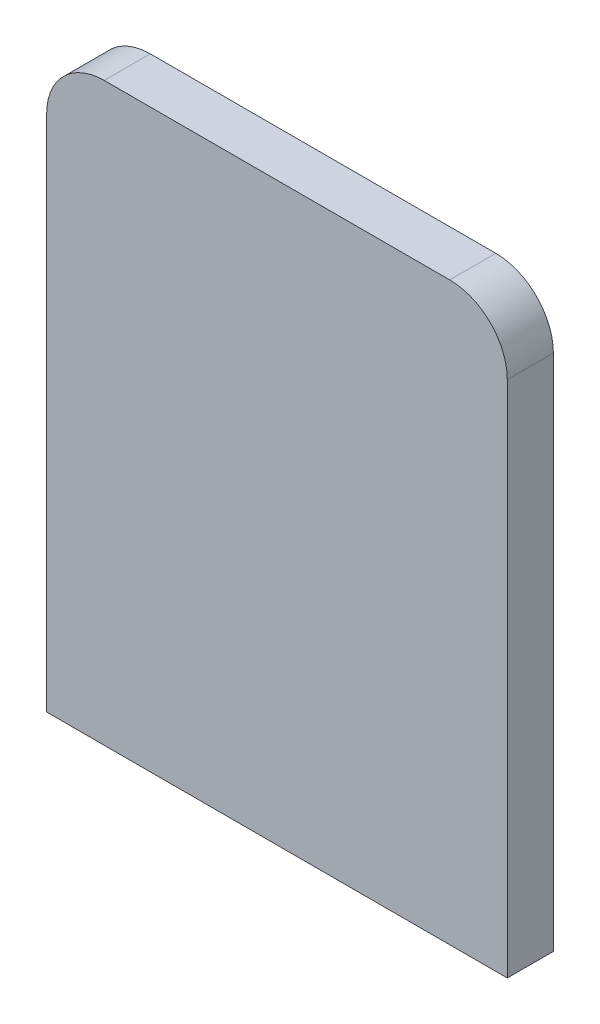
from build123d import *

# Parameters (mm, degrees)
SKETCH1_W           = 80
SKETCH1_H           = 100
BOSS_EXTRUDE1_DEPTH = 8
FILLET1_R           = 10


with BuildPart() as part:
    # Sketch1 → Boss-Extrude1 (new body)
    with BuildSketch(Plane.XY):
        with Locations((40, -50)):
            Rectangle(SKETCH1_W, SKETCH1_H)
    extrude(amount=BOSS_EXTRUDE1_DEPTH)

    # Fillet1
    fillet1_edges = [part.edges().sort_by_distance(p)[0] for p in [
        (0, 0, 4),
        (80, 0, 4),
    ]]
    fillet(fillet1_edges, radius=FILLET1_R)


solid = part.part
